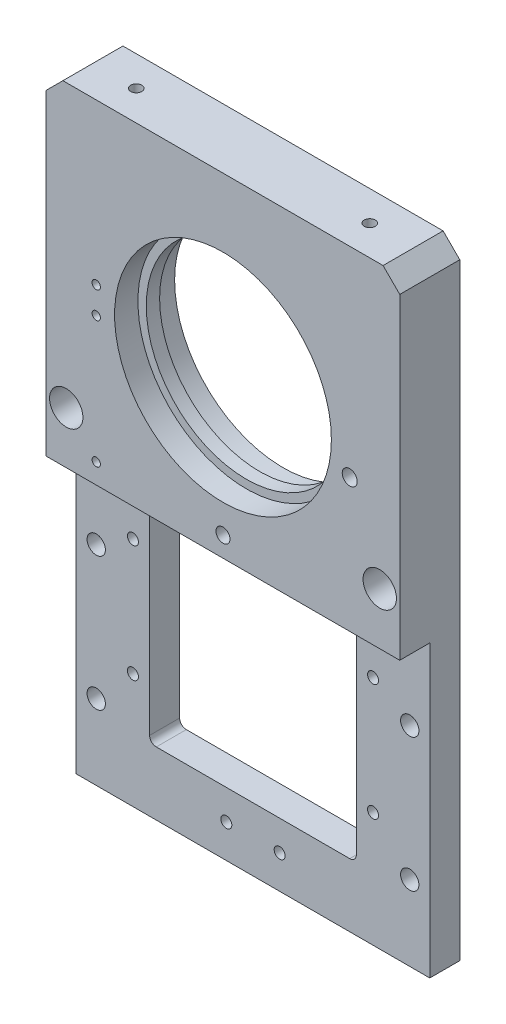
from build123d import *

# Parameters (mm, degrees)
SKETCH1_W                                            = 106
SKETCH1_H                                            = 187
BOSS_EXTRUDE1_DEPTH                                  = 9
SKETCH2_R                                            = 30
CUT_EXTRUDE1_DEPTH                                   = 109.973620661
SKETCH3_R                                            = 32.5
CUT_EXTRUDE2_DEPTH                                   = 7
CUT_EXTRUDE3_START                                   = -7
SKETCH4_R                                            = 32.5
CUT_EXTRUDE3_DEPTH                                   = 7
SKETCH5_W                                            = 62
SKETCH5_H                                            = 68
CUT_EXTRUDE4_DEPTH                                   = 109.973620661
FILLET1_R                                            = 2
SKETCH6_W                                            = 9
SKETCH6_H                                            = 87
CUT_EXTRUDE5_DEPTH                                   = 142.630681704
M4_TAPPED_HOLE1_D                                    = 3.3
M4_TAPPED_HOLE2_D                                    = 3.3
M3_TAPPED_HOLE1_D                                    = 2.5
M3_TAPPED_HOLE1_DEPTH                                = 7.5
M3_TAPPED_HOLE1_TIP                                  = 0.751075774
CHAMFER1_SIZE                                        = 5
HOLE_SIZE_PER_SOCKET_HEAD_CAP_SCREW_TYPE_D           = 4.5
HOLE_SIZE_PER_SOCKET_HEAD_CAP_SCREW_TYPE_CBORE_D     = 8
HOLE_SIZE_PER_SOCKET_HEAD_CAP_SCREW_TYPE_CBORE_DEPTH = 5
HOLE_SIZE_PER_SOCKET_HEAD_CAP_SCREW_2_D              = 5.5
HOLE_SIZE_PER_SOCKET_HEAD_CAP_SCREW_2_CBORE_D        = 10
HOLE_SIZE_PER_SOCKET_HEAD_CAP_SCREW_2_CBORE_DEPTH    = 9
M5_TAPPED_HOLE1_D                                    = 4.2
M5_TAPPED_HOLE1_DEPTH                                = 12.4
M5_TAPPED_HOLE1_TIP                                  = 1.2618073
M4_TAPPED_HOLE3_D                                    = 3.3
M4_TAPPED_HOLE3_DEPTH                                = 12.1
M4_TAPPED_HOLE3_TIP                                  = 0.991420021


with BuildPart() as part:
    # Sketch1 → Boss-Extrude1 (new, symmetric)
    with BuildSketch(Plane.XY):
        Rectangle(SKETCH1_W, SKETCH1_H)
    extrude(amount=BOSS_EXTRUDE1_DEPTH, both=True)

    # Sketch2 → Cut-Extrude1 (cut, through all)
    with BuildSketch(Plane(origin=(0, 0, -9), x_dir=(-1, 0, 0), z_dir=(0, 0, -1))):
        with Locations((0, 40.5)):
            Circle(SKETCH2_R)
    extrude(amount=-CUT_EXTRUDE1_DEPTH, mode=Mode.SUBTRACT)

    # Sketch3 → Cut-Extrude2 (cut)
    with BuildSketch(Plane.XY.offset(9)):
        with Locations((0, 40.5)):
            Circle(SKETCH3_R)
    extrude(amount=-CUT_EXTRUDE2_DEPTH, mode=Mode.SUBTRACT)

    # Sketch4 → Cut-Extrude3 (cut)
    with BuildSketch(Plane(origin=(0, 0, -9), x_dir=(-1, 0, 0), z_dir=(0, 0, -1)).offset(CUT_EXTRUDE3_START)):
        with Locations(Location((0, 40.5, 0), (0, 0, 180))):
            Circle(SKETCH4_R)
    extrude(amount=CUT_EXTRUDE3_DEPTH, mode=Mode.SUBTRACT)

    # Sketch5 → Cut-Extrude4 (cut, through all)
    with BuildSketch(Plane.XY.offset(9)):
        with Locations((0, -40.5)):
            Rectangle(SKETCH5_W, SKETCH5_H)
    extrude(amount=-CUT_EXTRUDE4_DEPTH, mode=Mode.SUBTRACT)

    # Fillet1
    fillet1_edges = [part.edges().sort_by_distance(p)[0] for p in [
        (-31, -74.5, 0),
        (-31, -6.5, 0),
        (31, -6.5, 0),
        (31, -74.5, 0),
    ]]
    fillet(fillet1_edges, radius=FILLET1_R)

    # Sketch6 → Cut-Extrude5 (cut, through all)
    with BuildSketch(Plane(origin=(53, 0, 0), x_dir=(0, 0, -1), z_dir=(1, 0, 0))):
        with Locations((-4.5, -50)):
            Rectangle(SKETCH6_W, SKETCH6_H)
    extrude(amount=-CUT_EXTRUDE5_DEPTH, mode=Mode.SUBTRACT)

    # M4 Tapped Hole1 (through all)
    with Locations(Plane.XY):
        with Locations((36, -24), (36, -59), (-36, -59), (-36, -24)):
            Hole(M4_TAPPED_HOLE1_D / 2)

    # M4 Tapped Hole2 (through all)
    with Locations(Plane.XY):
        with Locations((-8, -83.5), (8, -83.5)):
            Hole(M4_TAPPED_HOLE2_D / 2)

    # M3 Tapped Hole1
    with Locations(Plane.XY.offset(9)):
        with Locations((-38, 45.5), (-38, 37.5), (-38, -0.5)):
            Hole(M3_TAPPED_HOLE1_D / 2, depth=M3_TAPPED_HOLE1_DEPTH)
            with Locations((0, 0, -(M3_TAPPED_HOLE1_DEPTH + M3_TAPPED_HOLE1_TIP / 2))):  # 118° drill point
                Cone(0, M3_TAPPED_HOLE1_D / 2, M3_TAPPED_HOLE1_TIP, mode=Mode.SUBTRACT)

    # Chamfer1
    chamfer1_edges = [part.edges().sort_by_distance(p)[0] for p in [
        (-53, 93.5, 0),
        (53, 93.5, 0),
    ]]
    chamfer(chamfer1_edges, length=CHAMFER1_SIZE)

    # Hole size per socket head cap screw type (through all)
    with Locations(Plane(origin=(0, 0, -9), x_dir=(-1, 0, 0), z_dir=(0, 0, -1))):
        with Locations((-38, 33.5)):
            CounterBoreHole(HOLE_SIZE_PER_SOCKET_HEAD_CAP_SCREW_TYPE_D / 2, HOLE_SIZE_PER_SOCKET_HEAD_CAP_SCREW_TYPE_CBORE_D / 2, HOLE_SIZE_PER_SOCKET_HEAD_CAP_SCREW_TYPE_CBORE_DEPTH)

    # Hole size per socket head cap screw  2 (through all)
    with Locations(Plane.XY.offset(9)):
        with Locations((-47, 9.05741234), (-47, -30.94258766), (-47, -70.94258766), (47, -70.94258766), (47, -30.94258766), (47, 9.05741234)):
            CounterBoreHole(HOLE_SIZE_PER_SOCKET_HEAD_CAP_SCREW_2_D / 2, HOLE_SIZE_PER_SOCKET_HEAD_CAP_SCREW_2_CBORE_D / 2, HOLE_SIZE_PER_SOCKET_HEAD_CAP_SCREW_2_CBORE_DEPTH)

    # M5 Tapped Hole1
    with Locations(Plane.XY.offset(9)):
        with Locations((0, -0.5)):
            Hole(M5_TAPPED_HOLE1_D / 2, depth=M5_TAPPED_HOLE1_DEPTH)
            with Locations((0, 0, -(M5_TAPPED_HOLE1_DEPTH + M5_TAPPED_HOLE1_TIP / 2))):  # 118° drill point
                Cone(0, M5_TAPPED_HOLE1_D / 2, M5_TAPPED_HOLE1_TIP, mode=Mode.SUBTRACT)

    # M4 Tapped Hole3
    with Locations(Plane(origin=(0, 93.5, 0), x_dir=(1, 0, 0), z_dir=(0, 1, 0))):
        with Locations((-35, 0), (35, 0)):
            Hole(M4_TAPPED_HOLE3_D / 2, depth=M4_TAPPED_HOLE3_DEPTH)
            with Locations((0, 0, -(M4_TAPPED_HOLE3_DEPTH + M4_TAPPED_HOLE3_TIP / 2))):  # 118° drill point
                Cone(0, M4_TAPPED_HOLE3_D / 2, M4_TAPPED_HOLE3_TIP, mode=Mode.SUBTRACT)


solid = part.part
